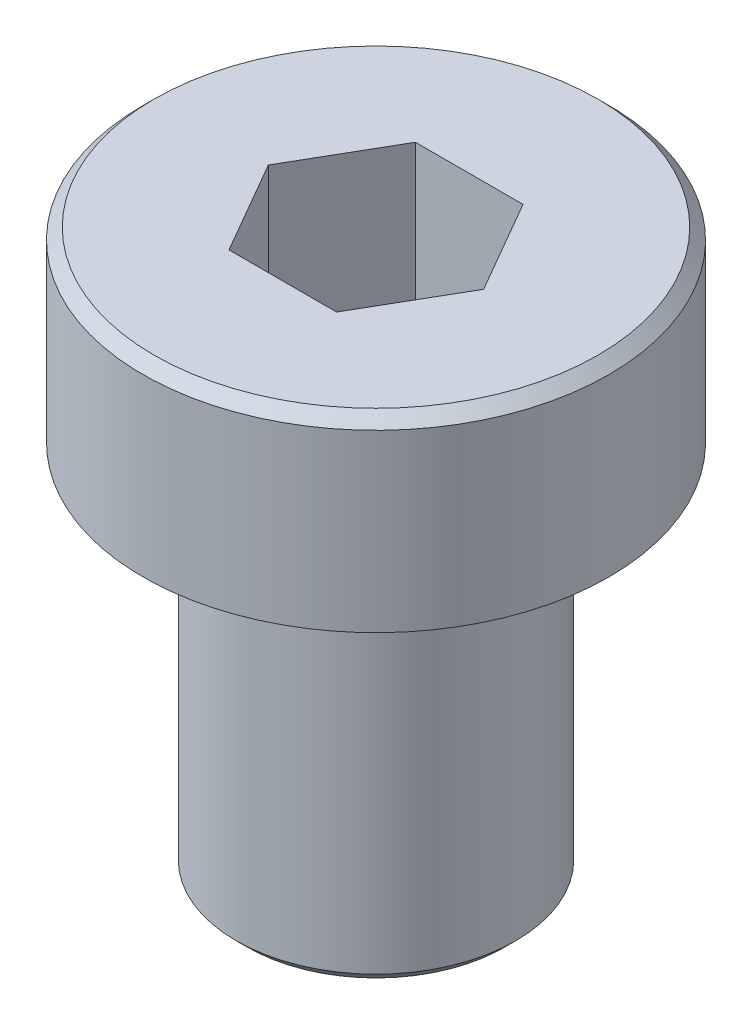
from build123d import *

# Parameters (mm, degrees)
CHAMFER1_SIZE         = 0.24
CUT_EXTRUDE1_DEPTH    = 3
BODY_MOVE_COPY1_ANGLE = 180


with BuildPart() as part:
    # Sketch2 → Revolve1 (revolve)
    with BuildSketch(Plane.XY):
        Polygon((2, -4), (2, -1), (0, 0.154700538), (0, 8), (3, 8), (3, 0), (5, 0), (5, -4), align=None)
    revolve(axis=Axis((0, 0.154700538, 0), (0, 1, 0)))

    # Chamfer1
    chamfer1_edges = [part.edges().sort_by_distance(p)[0] for p in [
        (-5, -4, 0),
        (-3, 8, 0),
    ]]
    chamfer(chamfer1_edges, length=CHAMFER1_SIZE)

    # Sketch3 → Cut-Extrude1 (cut)
    with BuildSketch(Plane.XZ.offset(4)):
        Polygon((-1.154700538, 2), (-2.309401077, 0), (-1.154700538, -2), (1.154700538, -2), (2.309401077, 0), (1.154700538, 2), align=None)
    extrude(amount=-CUT_EXTRUDE1_DEPTH, mode=Mode.SUBTRACT)


with BuildPart() as part_1:
    # Body-Move/Copy1: moved
    add(part.part.rotate(Axis((0, 3.25, 0), (1, 0, 0)), BODY_MOVE_COPY1_ANGLE))


solid = part_1.part
